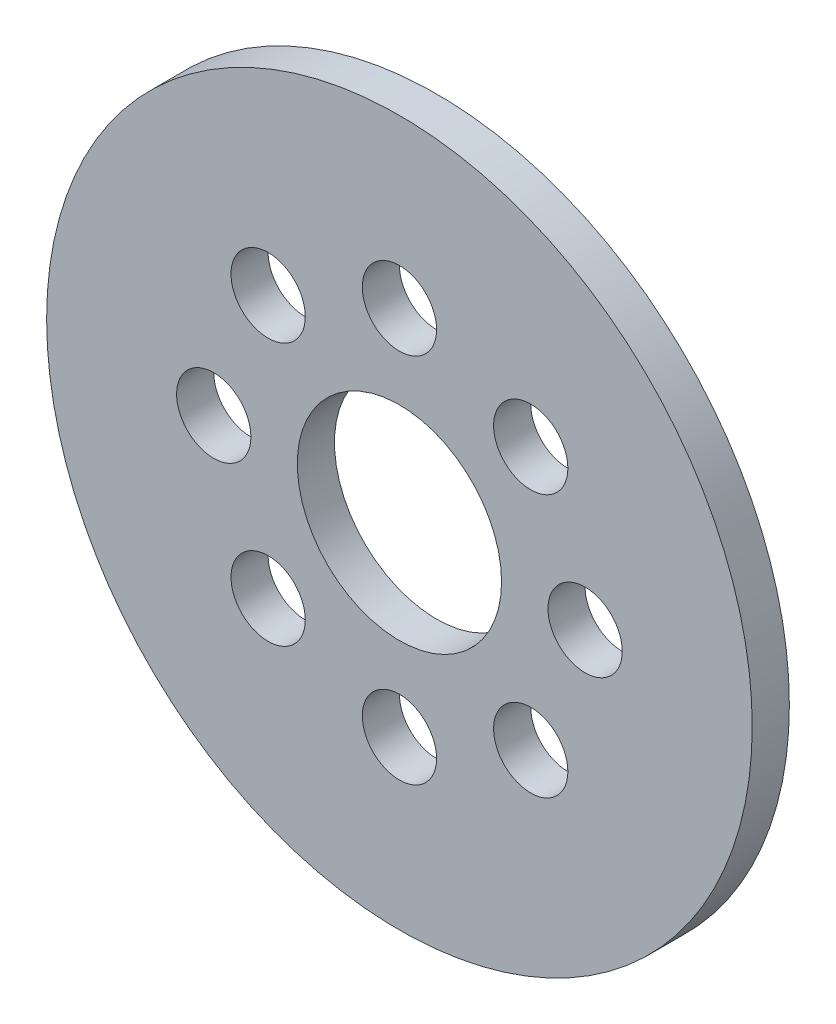
from build123d import *

# Parameters (mm, degrees)
SKETCH2_R           = 95
SKETCH2_R_2         = 27.5
BOSS_EXTRUDE1_DEPTH = 10
SKETCH3_R           = 10
CUT_EXTRUDE1_DEPTH  = 135.721935853
CIRPATTERN1_COUNT   = 8


with BuildPart() as part:
    # Sketch2 → Boss-Extrude1 (new body)
    with BuildSketch(Plane.XY):
        Circle(SKETCH2_R)
        Circle(SKETCH2_R_2, mode=Mode.SUBTRACT)
    extrude(amount=BOSS_EXTRUDE1_DEPTH)

    # Sketch3 → Cut-Extrude1 (cut, symmetric)
    with BuildSketch(Plane.XY.offset(10)):
        with Locations((50, 0)):
            Circle(SKETCH3_R)
    cut_extrude1 = extrude(amount=CUT_EXTRUDE1_DEPTH, both=True, mode=Mode.SUBTRACT)

    # CirPattern1: Cut-Extrude1 ×8 about axis
    cirpattern1_axis = Axis((0, 0, 0), (0, 0, 1))
    for i in range(1, CIRPATTERN1_COUNT):
        add(cut_extrude1.rotate(cirpattern1_axis, i * 360 / CIRPATTERN1_COUNT), mode=Mode.SUBTRACT)


solid = part.part
